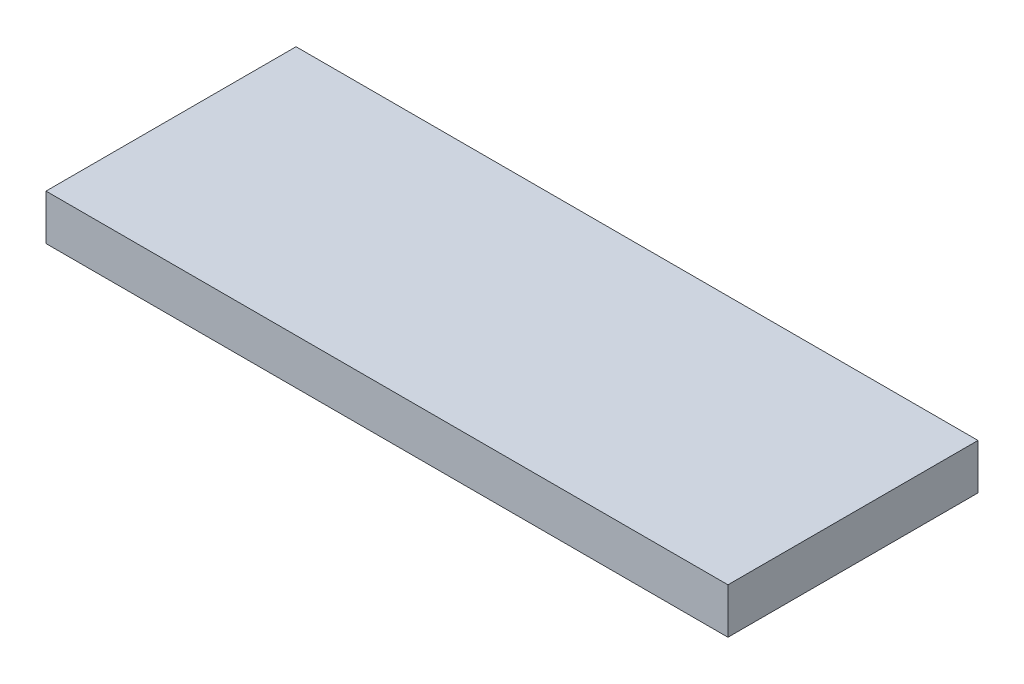
SolidWorks part; units mm, degrees
ref_plane "前视基准面" through (0, 0, 0) normal (0, 0, 1) x (1, 0, 0)
ref_plane "上视基准面" through (0, 0, 0) normal (0, 1, 0) x (1, 0, 0)
ref_plane "右视基准面" through (0, 0, 0) normal (1, 0, 0) x (0, 0, -1)
sketch "草图1" plane through (0, 0, 0) normal (0, 0, 1) x (1, 0, 0)
  line L1 (-75, -5) -> (75, -5)
  line L2 (-75, -5) -> (-75, 5)
  line L3 (-75, 5) -> (75, 5)
  line L4 (75, -5) -> (75, 5)
  line L5 (-75, -5) -> (75, 5) construction
  line L6 (-75, 5) -> (75, -5) construction
  point P0 (0, 0)
  dimension "D1" = 150
  dimension "D2" = 10
extrude "凸台-拉伸1" add sketch "草图1" along normal blind 55
